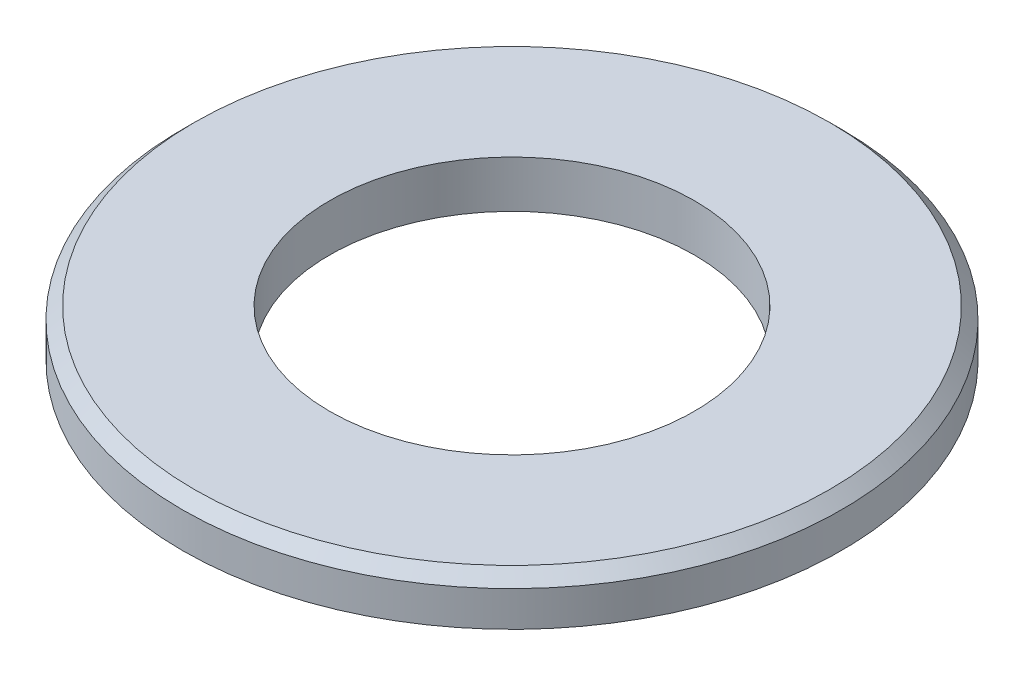
SolidWorks part; units mm, degrees
ref_plane "基准面1" through (0, 0, 0) normal (0, 0, 1) x (1, 0, 0)
ref_plane "基准面2" through (0, 0, 0) normal (0, 1, 0) x (1, 0, 0)
ref_plane "基准面3" through (0, 0, 0) normal (1, 0, 0) x (0, 0, -1)
sketch "尺寸草图" plane through (0, 0, 0) normal (0, 0, 1) x (1, 0, 0)
  line L0 (0, 0) -> (56, 0) construction
  point P3 (4, 0)
  point P4 (56, 0)
  point P5 (31, 0)
  dimension "h" = 4
  dimension "d2" = 56
  dimension "d1" = 31
sketch "草图1" plane through (0, 0, 0) normal (0, 0, 1) x (1, 0, 0)
  line L0 (0, 0) -> (0, 52.7318) construction
  line L1 (-27, 12.6445) -> (-28, 11.6445)
  line L2 (-15.5, 8.6445) -> (-28, 8.6445)
  line L3 (-15.5, 8.6445) -> (-15.5, 12.6445)
  line L4 (-15.5, 12.6445) -> (-27, 12.6445)
  line L5 (-28, 8.6445) -> (-28, 11.6445)
  point P4 (-28, 12.6445)
  dimension "D1" = 15.5
  dimension "D2" = 28
  dimension "h" = 4
revolve "基体-旋转" add sketch "草图1" angle 360 about L0
